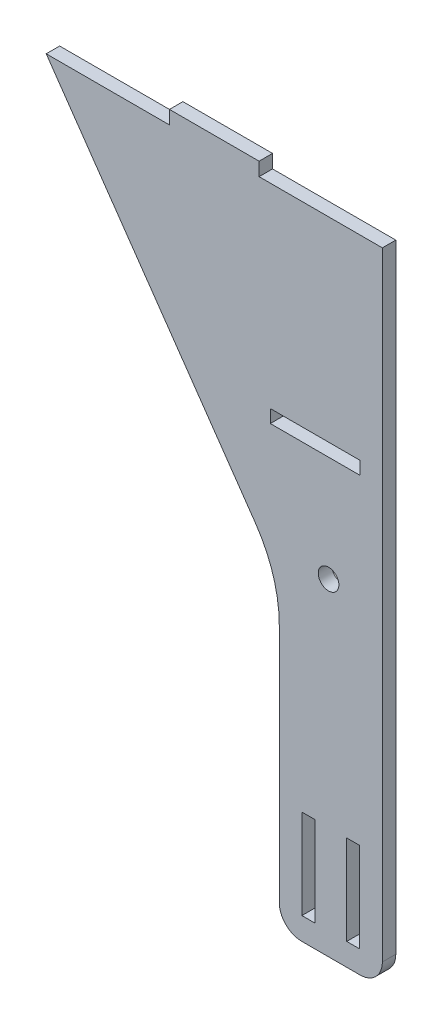
from build123d import *

# Parameters (mm, degrees)
SKETCH1_W           = 2.9
SKETCH1_H           = 20
BOSS_EXTRUDE1_DEPTH = 3
FILLET1_R           = 5
FILLET2_R           = 30
SKETCH4_R           = 2.3
CUT_EXTRUDE1_DEPTH  = 10
SKETCH5_W           = 20
SKETCH5_H           = 2.9
CUT_EXTRUDE2_DEPTH  = 165.164551594


with BuildPart() as part:
    # Sketch1 → Boss-Extrude1 (new body)
    with BuildSketch(Plane.XY):
        Polygon((0, 0), (-23, 0), (-23, 68), (-75, 143), (-47.5, 143), (-47.5, 146), (-27.5, 146), (-27.5, 143), (0, 143), align=None)
        with Locations((-16.5, 15)):
            Rectangle(SKETCH1_W, SKETCH1_H, mode=Mode.SUBTRACT)
        with Locations((-6.5, 15)):
            Rectangle(SKETCH1_W, SKETCH1_H, mode=Mode.SUBTRACT)
    extrude(amount=BOSS_EXTRUDE1_DEPTH)

    # Fillet1
    fillet1_edges = [part.edges().sort_by_distance(p)[0] for p in [
        (0, 0, 1.5),
        (-23, 0, 1.5),
    ]]
    fillet(fillet1_edges, radius=FILLET1_R)

    # Fillet2
    fillet2_edges = [part.edges().sort_by_distance(p)[0] for p in [
        (-23, 68, 1.5),
    ]]
    fillet(fillet2_edges, radius=FILLET2_R)

    # Sketch4 → Cut-Extrude1 (cut)
    with BuildSketch(Plane.XY.offset(3)):
        with Locations((-12, 73)):
            Circle(SKETCH4_R)
    extrude(amount=-CUT_EXTRUDE1_DEPTH, mode=Mode.SUBTRACT)

    # Sketch5 → Cut-Extrude2 (cut, through all)
    with BuildSketch(Plane(origin=(0, 0, 0), x_dir=(-1, 0, 0), z_dir=(0, 0, -1))):
        with Locations((15, 98)):
            Rectangle(SKETCH5_W, SKETCH5_H)
    extrude(amount=-CUT_EXTRUDE2_DEPTH, mode=Mode.SUBTRACT)


solid = part.part
